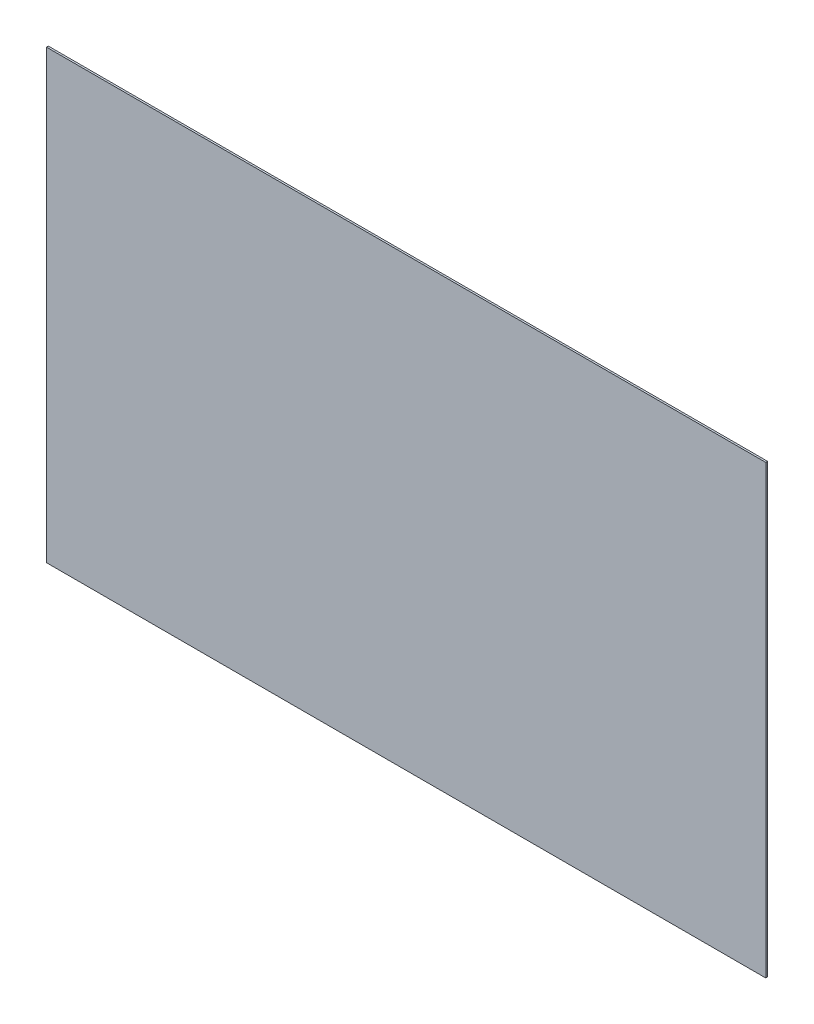
from build123d import *

# Parameters (mm, degrees)
SKETCH_1_W      = 1160
SKETCH_1_H      = 720
EXTRUDE_1_DEPTH = 3


with BuildPart() as part:
    # 草图1 → 凸台-拉伸1 (new body)
    with BuildSketch(Plane.XY):
        Rectangle(SKETCH_1_W, SKETCH_1_H)
    extrude(amount=EXTRUDE_1_DEPTH)


solid = part.part
